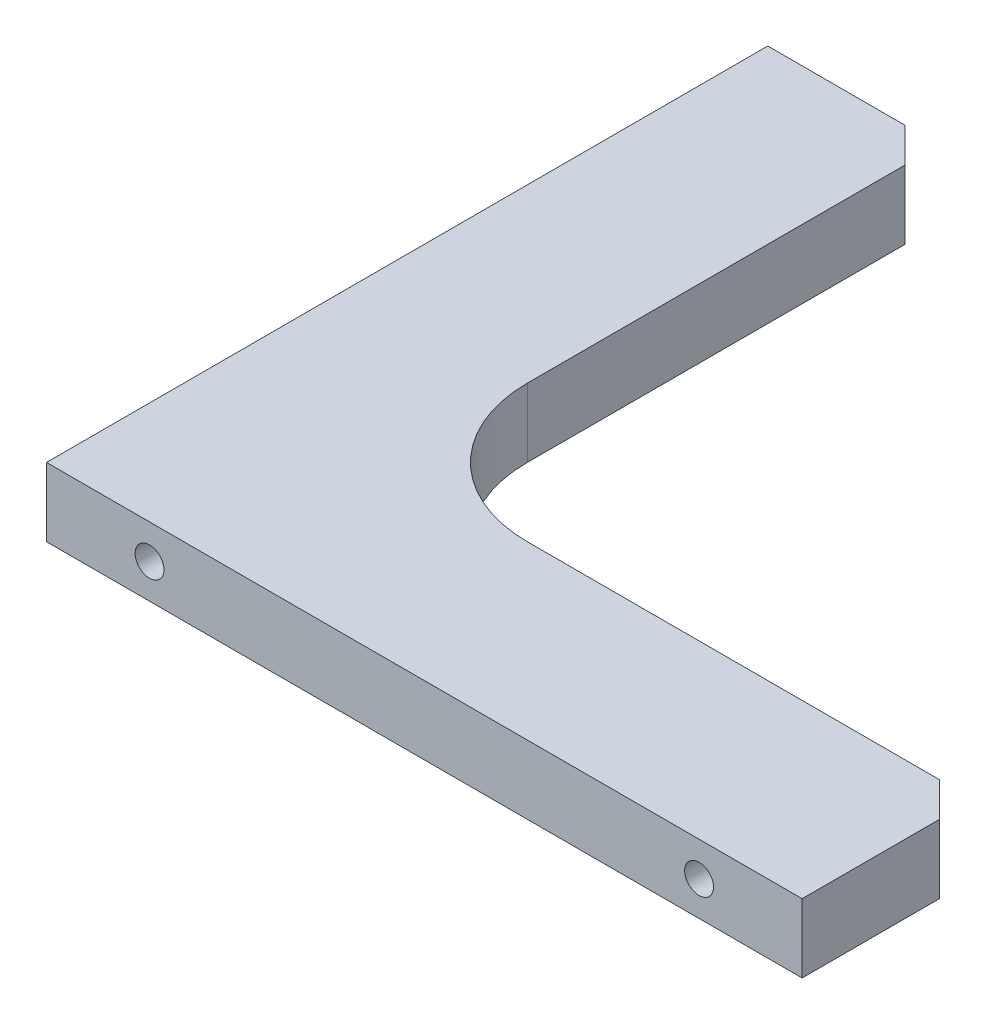
SolidWorks part; units mm, degrees
material "A6061"
ref_plane "前基準面" through (0, 0, 0) normal (0, 0, 1) x (1, 0, 0)
ref_plane "上基準面" through (0, 0, 0) normal (0, 1, 0) x (1, 0, 0)
ref_plane "右基準面" through (0, 0, 0) normal (1, 0, 0) x (0, 0, -1)
sketch "草图1" plane through (0, 0, 0) normal (0, 1, 0) x (1, 0, 0)
  line L1 (-55, -52.5) -> (55, -52.5)
  line L2 (-55, -52.5) -> (-55, 52.5)
  line L3 (-55, 52.5) -> (55, 52.5)
  line L4 (55, -52.5) -> (55, 52.5)
  line L5 (-55, -52.5) -> (55, 52.5) construction
  line L6 (-55, 52.5) -> (55, -52.5) construction
  point P0 (0, 0)
  dimension "D1" = 110
  dimension "D2" = 105
extrude "凸台-拉伸1" add sketch "草图1" along normal mid plane 10
sketch "草图2" plane through (0, 5, 0) normal (0, 1, 0) x (1, 0, 0)
  line L0 (-55, -52.5) -> (55, -52.5) construction
  line L1 (55, 52.5) -> (-30, 52.5)
  line L2 (55, 52.5) -> (55, -27.5)
  line L3 (55, -27.5) -> (-10, -27.5)
  line L4 (-30, 52.5) -> (-30, -7.5)
  line L5 (-55, 52.5) -> (-55, -52.5) construction
  arc A0 (-10, -27.5) -> (-30, -7.5) centre (-10, -7.5) cw
  dimension "D3" = 20
  dimension "D1" = 25
  dimension "D2" = 25
extrude "切除-拉伸1" cut sketch "草图2" against normal up to surface (10 mm away) up to face at (0, -5, 0)
chamfer "倒角1" distance 5 angle 45 2 edges at (-30, 0, -52.5) (55, 0, 27.5)
hole_wizard "M5 螺纹孔1" positions "草图3" profile "草图4" tap size "M5" standard "GB"
sketch "草图3" plane through (-55, 0, 0) normal (-1, 0, 0) x (0, 0, 1)
  line L0 (52.5, 5) -> (52.5, -5) construction
  point P0 (37.5, 0)
  point P2 (-42.5, 0)
  dimension "D1" = 15
  dimension "D2" = 80
sketch "草图4" plane through (-55, 0, 37.5) normal (0, 1, 0) x (0, 0, 1)
  line L0 (0, 0) -> (0, 13.6618)
  line L1 (0, 13.6618) -> (2.1, 12.4)
  line L2 (2.1, 12.4) -> (2.1, 0)
  line L5 (2.1, 0) -> (0, 0)
  line L10 (0, 13.6618) -> (-2.1, 12.4) construction
  line L11 (0, -6.35) -> (0, 107.95) construction
  dimension "螺纹孔钻头直径" = 4.2
  dimension "螺纹孔钻头深度" = 12.4
  dimension "导头角度" = 118
cosmetic thread "孔螺蚊线1" parameters "D1"=10, "D2"=5
cosmetic thread "孔螺蚊线2" parameters "D1"=10, "D2"=5
ref_plane "基准面1" through (-1.25, 0, -1.25) normal (-0.7071, 0, -0.7071) x (-0.7071, 0, 0.7071)
mirror "镜向1" about plane through (-1.25, 0, -1.25) normal (-0.7071, 0, -0.7071) of "M5 螺纹孔1"
